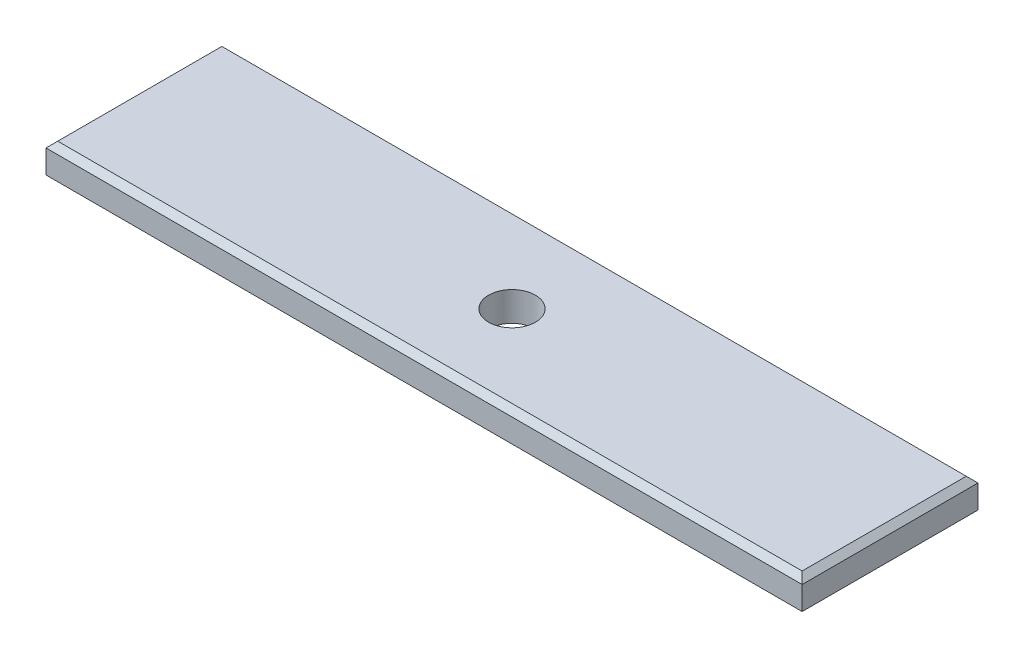
SolidWorks part; units mm, degrees
ref_plane "Front Plane" through (0, 0, 0) normal (0, 0, 1) x (1, 0, 0)
ref_plane "Top Plane" through (0, 0, 0) normal (0, 1, 0) x (1, 0, 0)
ref_plane "Right Plane" through (0, 0, 0) normal (1, 0, 0) x (0, 0, -1)
sketch "Sketch1" plane through (0, 0, 0) normal (0, 1, 0) x (1, 0, 0)
  line L1 (-64.5, -15) -> (64.5, -15)
  line L2 (-64.5, -15) -> (-64.5, 15)
  line L3 (-64.5, 15) -> (64.5, 15)
  line L4 (64.5, -15) -> (64.5, 15)
  line L5 (-64.5, -15) -> (64.5, 15) construction
  line L6 (-64.5, 15) -> (64.5, -15) construction
  point P0 (0, 0)
  dimension "D1" = 129
  dimension "D2" = 30
extrude "Boss-Extrude1" add sketch "Sketch1" along normal blind 5
sketch "Sketch3" plane through (0, 5, 0) normal (0, 1, 0) x (1, 0, 0)
  circle A0 centre (0, 0) radius 4
  dimension "D1" = 8
extrude "Cut-Extrude1" cut sketch "Sketch3" against normal up to next
chamfer "Chamfer1" distance 1 angle 45 4 edges at (64.5, 5, 0) (0, 5, 15) (-64.5, 5, 0) (0, 5, -15)
